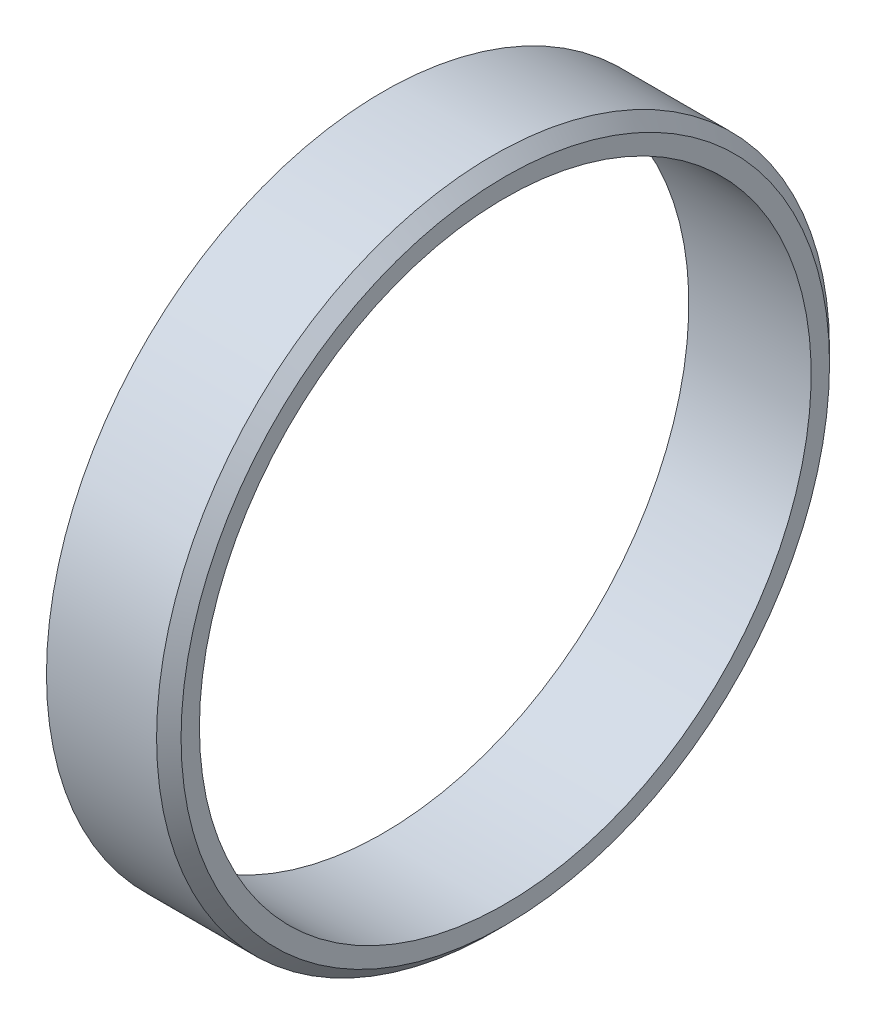
SolidWorks part; units mm, degrees
material "黄铜"
ref_plane "前视基准面" through (0, 0, 0) normal (0, 0, 1) x (1, 0, 0)
ref_plane "上视基准面" through (0, 0, 0) normal (0, 1, 0) x (1, 0, 0)
ref_plane "右视基准面" through (0, 0, 0) normal (1, 0, 0) x (0, 0, -1)
other "Configuration Table"
sketch "草图1" plane through (0, 0, 0) normal (0, 1, 0) x (1, 0, 0)
  line L0 (-308.2128, 0) -> (15102.4271, 0) construction
  line L1 (0, 25) -> (0, 27.5)
  line L4 (0, 27.5) -> (10, 27.5)
  line L5 (10, 27.5) -> (10, 25)
  line L6 (10, 25) -> (0, 25)
  point P6 (0, 27.5)
  point P9 (2.7966, 11.3136)
  point P10 (0.1465, 27.5)
  dimension "D1" = 10
  dimension "D3" = 50
  dimension "D4" = 55
revolve "旋转1" add sketch "草图1" angle 360 about L0
chamfer "倒角1" distance 1 angle 45 1 edges at (10, 0, 27.5)
